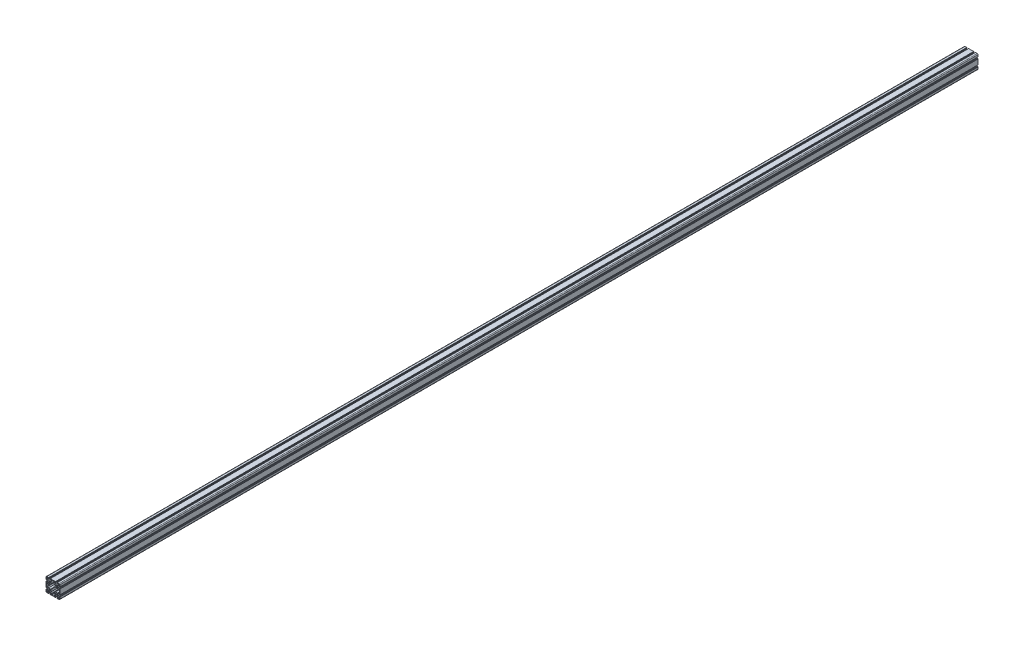
from build123d import *

# Parameters (mm, degrees)
SKETCH1_R           = 3.4
BOSS_EXTRUDE1_DEPTH = 5338


with BuildPart() as part:
    # Sketch1 → Boss-Extrude1 (new body)
    with BuildSketch(Plane.XY.offset(100)):
        with BuildLine():
            Line((37.78472507, 10.370402299), (32.802492023, 10.370402299))
            Line((32.802492023, 10.370402299), (28.48472507, 14.688169252))
            Line((28.48472507, 14.688169252), (28.48472507, 26.552635346))
            Line((28.48472507, 26.552635346), (32.802492023, 30.870402299))
            Line((32.802492023, 30.870402299), (37.78472507, 30.870402299))
            ThreePointArc((37.78472507, 30.870402299), (38.491831851, 30.57750908), (38.78472507, 29.870402299))
            Line((38.78472507, 29.870402299), (38.78472507, 28.220402299))
            ThreePointArc((38.78472507, 28.220402299), (38.491831851, 27.513295518), (37.78472507, 27.220402299))
            Line((37.78472507, 27.220402299), (36.28472507, 27.220402299))
            Line((36.28472507, 27.220402299), (36.28472507, 25.020402299))
            ThreePointArc((36.28472507, 25.020402299), (36.372593036, 24.808270264), (36.58472507, 24.720402299))
            Line((36.58472507, 24.720402299), (39.78472507, 24.720402299))
            Line((39.78472507, 24.720402299), (39.78472507, 25.520402299))
            ThreePointArc((39.78472507, 25.520402299), (39.843303714, 25.661823655), (39.98472507, 25.720402299))
            Line((39.98472507, 25.720402299), (40.78472507, 25.720402299))
            Line((40.78472507, 25.720402299), (40.78472507, 36.120402299))
            ThreePointArc((40.78472507, 36.120402299), (39.466705585, 39.302382814), (36.28472507, 40.620402299))
            Line((36.28472507, 40.620402299), (25.88472507, 40.620402299))
            Line((25.88472507, 40.620402299), (25.88472507, 39.820402299))
            ThreePointArc((25.88472507, 39.820402299), (25.826146426, 39.678980943), (25.68472507, 39.620402299))
            Line((25.68472507, 39.620402299), (24.88472507, 39.620402299))
            Line((24.88472507, 39.620402299), (24.88472507, 36.420402299))
            ThreePointArc((24.88472507, 36.420402299), (24.972593036, 36.208270264), (25.18472507, 36.120402299))
            Line((25.18472507, 36.120402299), (27.38472507, 36.120402299))
            Line((27.38472507, 36.120402299), (27.38472507, 37.620402299))
            ThreePointArc((27.38472507, 37.620402299), (27.677618289, 38.32750908), (28.38472507, 38.620402299))
            Line((28.38472507, 38.620402299), (30.03472507, 38.620402299))
            ThreePointArc((30.03472507, 38.620402299), (30.741831851, 38.32750908), (31.03472507, 37.620402299))
            Line((31.03472507, 37.620402299), (31.03472507, 32.638169252))
            Line((31.03472507, 32.638169252), (26.716958117, 28.320402299))
            Line((26.716958117, 28.320402299), (14.852492023, 28.320402299))
            Line((14.852492023, 28.320402299), (10.53472507, 32.638169252))
            Line((10.53472507, 32.638169252), (10.53472507, 37.620402299))
            ThreePointArc((10.53472507, 37.620402299), (10.827618289, 38.32750908), (11.53472507, 38.620402299))
            Line((11.53472507, 38.620402299), (13.18472507, 38.620402299))
            ThreePointArc((13.18472507, 38.620402299), (13.891831851, 38.32750908), (14.18472507, 37.620402299))
            Line((14.18472507, 37.620402299), (14.18472507, 36.120402299))
            Line((14.18472507, 36.120402299), (16.38472507, 36.120402299))
            ThreePointArc((16.38472507, 36.120402299), (16.596857104, 36.208270264), (16.68472507, 36.420402299))
            Line((16.68472507, 36.420402299), (16.68472507, 39.620402299))
            Line((16.68472507, 39.620402299), (15.88472507, 39.620402299))
            ThreePointArc((15.88472507, 39.620402299), (15.743303714, 39.678980943), (15.68472507, 39.820402299))
            Line((15.68472507, 39.820402299), (15.68472507, 40.620402299))
            Line((15.68472507, 40.620402299), (-14.11527493, 40.620402299))
            Line((-14.11527493, 40.620402299), (-14.11527493, 39.820402299))
            ThreePointArc((-14.11527493, 39.820402299), (-14.173853574, 39.678980943), (-14.31527493, 39.620402299))
            Line((-14.31527493, 39.620402299), (-15.11527493, 39.620402299))
            Line((-15.11527493, 39.620402299), (-15.11527493, 36.420402299))
            ThreePointArc((-15.11527493, 36.420402299), (-15.027406964, 36.208270264), (-14.81527493, 36.120402299))
            Line((-14.81527493, 36.120402299), (-12.61527493, 36.120402299))
            Line((-12.61527493, 36.120402299), (-12.61527493, 37.620402299))
            ThreePointArc((-12.61527493, 37.620402299), (-12.322381711, 38.32750908), (-11.61527493, 38.620402299))
            Line((-11.61527493, 38.620402299), (-9.96527493, 38.620402299))
            ThreePointArc((-9.96527493, 38.620402299), (-9.258168149, 38.32750908), (-8.96527493, 37.620402299))
            Line((-8.96527493, 37.620402299), (-8.96527493, 32.638169252))
            Line((-8.96527493, 32.638169252), (-13.283041883, 28.320402299))
            Line((-13.283041883, 28.320402299), (-25.147507977, 28.320402299))
            Line((-25.147507977, 28.320402299), (-29.46527493, 32.638169252))
            Line((-29.46527493, 32.638169252), (-29.46527493, 37.620402299))
            ThreePointArc((-29.46527493, 37.620402299), (-29.172381711, 38.32750908), (-28.46527493, 38.620402299))
            Line((-28.46527493, 38.620402299), (-26.81527493, 38.620402299))
            ThreePointArc((-26.81527493, 38.620402299), (-26.108168149, 38.32750908), (-25.81527493, 37.620402299))
            Line((-25.81527493, 37.620402299), (-25.81527493, 36.120402299))
            Line((-25.81527493, 36.120402299), (-23.61527493, 36.120402299))
            ThreePointArc((-23.61527493, 36.120402299), (-23.403142896, 36.208270264), (-23.31527493, 36.420402299))
            Line((-23.31527493, 36.420402299), (-23.31527493, 39.620402299))
            Line((-23.31527493, 39.620402299), (-24.11527493, 39.620402299))
            ThreePointArc((-24.11527493, 39.620402299), (-24.256696286, 39.678980943), (-24.31527493, 39.820402299))
            Line((-24.31527493, 39.820402299), (-24.31527493, 40.620402299))
            Line((-24.31527493, 40.620402299), (-34.71527493, 40.620402299))
            ThreePointArc((-34.71527493, 40.620402299), (-37.897255445, 39.302382814), (-39.21527493, 36.120402299))
            Line((-39.21527493, 36.120402299), (-39.21527493, 25.720402299))
            Line((-39.21527493, 25.720402299), (-38.41527493, 25.720402299))
            ThreePointArc((-38.41527493, 25.720402299), (-38.273853574, 25.661823655), (-38.21527493, 25.520402299))
            Line((-38.21527493, 25.520402299), (-38.21527493, 24.720402299))
            Line((-38.21527493, 24.720402299), (-35.01527493, 24.720402299))
            ThreePointArc((-35.01527493, 24.720402299), (-34.803142896, 24.808270264), (-34.71527493, 25.020402299))
            Line((-34.71527493, 25.020402299), (-34.71527493, 27.220402299))
            Line((-34.71527493, 27.220402299), (-36.21527493, 27.220402299))
            ThreePointArc((-36.21527493, 27.220402299), (-36.922381711, 27.513295518), (-37.21527493, 28.220402299))
            Line((-37.21527493, 28.220402299), (-37.21527493, 29.870402299))
            ThreePointArc((-37.21527493, 29.870402299), (-36.922381711, 30.57750908), (-36.21527493, 30.870402299))
            Line((-36.21527493, 30.870402299), (-31.233041883, 30.870402299))
            Line((-31.233041883, 30.870402299), (-26.91527493, 26.552635346))
            Line((-26.91527493, 26.552635346), (-26.91527493, 14.688169252))
            Line((-26.91527493, 14.688169252), (-31.233041883, 10.370402299))
            Line((-31.233041883, 10.370402299), (-36.21527493, 10.370402299))
            ThreePointArc((-36.21527493, 10.370402299), (-36.922381711, 10.663295518), (-37.21527493, 11.370402299))
            Line((-37.21527493, 11.370402299), (-37.21527493, 13.020402299))
            ThreePointArc((-37.21527493, 13.020402299), (-36.922381711, 13.72750908), (-36.21527493, 14.020402299))
            Line((-36.21527493, 14.020402299), (-34.71527493, 14.020402299))
            Line((-34.71527493, 14.020402299), (-34.71527493, 16.220402299))
            ThreePointArc((-34.71527493, 16.220402299), (-34.803142896, 16.432534333), (-35.01527493, 16.520402299))
            Line((-35.01527493, 16.520402299), (-38.21527493, 16.520402299))
            Line((-38.21527493, 16.520402299), (-38.21527493, 15.720402299))
            ThreePointArc((-38.21527493, 15.720402299), (-38.273853574, 15.578980943), (-38.41527493, 15.520402299))
            Line((-38.41527493, 15.520402299), (-39.21527493, 15.520402299))
            Line((-39.21527493, 15.520402299), (-39.21527493, -14.279597701))
            Line((-39.21527493, -14.279597701), (-38.41527493, -14.279597701))
            ThreePointArc((-38.41527493, -14.279597701), (-38.273853574, -14.338176345), (-38.21527493, -14.479597701))
            Line((-38.21527493, -14.479597701), (-38.21527493, -15.279597701))
            Line((-38.21527493, -15.279597701), (-35.01527493, -15.279597701))
            ThreePointArc((-35.01527493, -15.279597701), (-34.803142896, -15.191729736), (-34.71527493, -14.979597701))
            Line((-34.71527493, -14.979597701), (-34.71527493, -12.779597701))
            Line((-34.71527493, -12.779597701), (-36.21527493, -12.779597701))
            ThreePointArc((-36.21527493, -12.779597701), (-36.922381711, -12.486704482), (-37.21527493, -11.779597701))
            Line((-37.21527493, -11.779597701), (-37.21527493, -10.129597701))
            ThreePointArc((-37.21527493, -10.129597701), (-36.922381711, -9.42249092), (-36.21527493, -9.129597701))
            Line((-36.21527493, -9.129597701), (-31.233041883, -9.129597701))
            Line((-31.233041883, -9.129597701), (-26.91527493, -13.447364654))
            Line((-26.91527493, -13.447364654), (-26.91527493, -25.311830748))
            Line((-26.91527493, -25.311830748), (-31.233041883, -29.629597701))
            Line((-31.233041883, -29.629597701), (-36.21527493, -29.629597701))
            ThreePointArc((-36.21527493, -29.629597701), (-36.922381711, -29.336704482), (-37.21527493, -28.629597701))
            Line((-37.21527493, -28.629597701), (-37.21527493, -26.979597701))
            ThreePointArc((-37.21527493, -26.979597701), (-36.922381711, -26.27249092), (-36.21527493, -25.979597701))
            Line((-36.21527493, -25.979597701), (-34.71527493, -25.979597701))
            Line((-34.71527493, -25.979597701), (-34.71527493, -23.779597701))
            ThreePointArc((-34.71527493, -23.779597701), (-34.803142896, -23.567465667), (-35.01527493, -23.479597701))
            Line((-35.01527493, -23.479597701), (-38.21527493, -23.479597701))
            Line((-38.21527493, -23.479597701), (-38.21527493, -24.279597701))
            ThreePointArc((-38.21527493, -24.279597701), (-38.273853574, -24.421019057), (-38.41527493, -24.479597701))
            Line((-38.41527493, -24.479597701), (-39.21527493, -24.479597701))
            Line((-39.21527493, -24.479597701), (-39.21527493, -34.879597701))
            ThreePointArc((-39.21527493, -34.879597701), (-37.897255445, -38.061578216), (-34.71527493, -39.379597701))
            Line((-34.71527493, -39.379597701), (-24.31527493, -39.379597701))
            Line((-24.31527493, -39.379597701), (-24.31527493, -38.579597701))
            ThreePointArc((-24.31527493, -38.579597701), (-24.256696286, -38.438176345), (-24.11527493, -38.379597701))
            Line((-24.11527493, -38.379597701), (-23.31527493, -38.379597701))
            Line((-23.31527493, -38.379597701), (-23.31527493, -35.179597701))
            ThreePointArc((-23.31527493, -35.179597701), (-23.403142896, -34.967465667), (-23.61527493, -34.879597701))
            Line((-23.61527493, -34.879597701), (-25.81527493, -34.879597701))
            Line((-25.81527493, -34.879597701), (-25.81527493, -36.379597701))
            ThreePointArc((-25.81527493, -36.379597701), (-26.108168149, -37.086704482), (-26.81527493, -37.379597701))
            Line((-26.81527493, -37.379597701), (-28.46527493, -37.379597701))
            ThreePointArc((-28.46527493, -37.379597701), (-29.172381711, -37.086704482), (-29.46527493, -36.379597701))
            Line((-29.46527493, -36.379597701), (-29.46527493, -31.397364654))
            Line((-29.46527493, -31.397364654), (-25.147507977, -27.079597701))
            Line((-25.147507977, -27.079597701), (-13.283041883, -27.079597701))
            Line((-13.283041883, -27.079597701), (-8.96527493, -31.397364654))
            Line((-8.96527493, -31.397364654), (-8.96527493, -36.379597701))
            ThreePointArc((-8.96527493, -36.379597701), (-9.258168149, -37.086704482), (-9.96527493, -37.379597701))
            Line((-9.96527493, -37.379597701), (-11.61527493, -37.379597701))
            ThreePointArc((-11.61527493, -37.379597701), (-12.322381711, -37.086704482), (-12.61527493, -36.379597701))
            Line((-12.61527493, -36.379597701), (-12.61527493, -34.879597701))
            Line((-12.61527493, -34.879597701), (-14.81527493, -34.879597701))
            ThreePointArc((-14.81527493, -34.879597701), (-15.027406964, -34.967465667), (-15.11527493, -35.179597701))
            Line((-15.11527493, -35.179597701), (-15.11527493, -38.379597701))
            Line((-15.11527493, -38.379597701), (-14.31527493, -38.379597701))
            ThreePointArc((-14.31527493, -38.379597701), (-14.173853574, -38.438176345), (-14.11527493, -38.579597701))
            Line((-14.11527493, -38.579597701), (-14.11527493, -39.379597701))
            Line((-14.11527493, -39.379597701), (15.68472507, -39.379597701))
            Line((15.68472507, -39.379597701), (15.68472507, -38.579597701))
            ThreePointArc((15.68472507, -38.579597701), (15.743303714, -38.438176345), (15.88472507, -38.379597701))
            Line((15.88472507, -38.379597701), (16.68472507, -38.379597701))
            Line((16.68472507, -38.379597701), (16.68472507, -35.179597701))
            ThreePointArc((16.68472507, -35.179597701), (16.596857104, -34.967465667), (16.38472507, -34.879597701))
            Line((16.38472507, -34.879597701), (14.18472507, -34.879597701))
            Line((14.18472507, -34.879597701), (14.18472507, -36.379597701))
            ThreePointArc((14.18472507, -36.379597701), (13.891831851, -37.086704482), (13.18472507, -37.379597701))
            Line((13.18472507, -37.379597701), (11.53472507, -37.379597701))
            ThreePointArc((11.53472507, -37.379597701), (10.827618289, -37.086704482), (10.53472507, -36.379597701))
            Line((10.53472507, -36.379597701), (10.53472507, -31.397364654))
            Line((10.53472507, -31.397364654), (14.852492023, -27.079597701))
            Line((14.852492023, -27.079597701), (26.716958117, -27.079597701))
            Line((26.716958117, -27.079597701), (31.03472507, -31.397364654))
            Line((31.03472507, -31.397364654), (31.03472507, -36.379597701))
            ThreePointArc((31.03472507, -36.379597701), (30.741831851, -37.086704482), (30.03472507, -37.379597701))
            Line((30.03472507, -37.379597701), (28.38472507, -37.379597701))
            ThreePointArc((28.38472507, -37.379597701), (27.677618289, -37.086704482), (27.38472507, -36.379597701))
            Line((27.38472507, -36.379597701), (27.38472507, -34.879597701))
            Line((27.38472507, -34.879597701), (25.18472507, -34.879597701))
            ThreePointArc((25.18472507, -34.879597701), (24.972593036, -34.967465667), (24.88472507, -35.179597701))
            Line((24.88472507, -35.179597701), (24.88472507, -38.379597701))
            Line((24.88472507, -38.379597701), (25.68472507, -38.379597701))
            ThreePointArc((25.68472507, -38.379597701), (25.826146426, -38.438176345), (25.88472507, -38.579597701))
            Line((25.88472507, -38.579597701), (25.88472507, -39.379597701))
            Line((25.88472507, -39.379597701), (36.28472507, -39.379597701))
            ThreePointArc((36.28472507, -39.379597701), (39.466705585, -38.061578216), (40.78472507, -34.879597701))
            Line((40.78472507, -34.879597701), (40.78472507, -24.479597701))
            Line((40.78472507, -24.479597701), (39.98472507, -24.479597701))
            ThreePointArc((39.98472507, -24.479597701), (39.843303714, -24.421019057), (39.78472507, -24.279597701))
            Line((39.78472507, -24.279597701), (39.78472507, -23.479597701))
            Line((39.78472507, -23.479597701), (36.58472507, -23.479597701))
            ThreePointArc((36.58472507, -23.479597701), (36.372593036, -23.567465667), (36.28472507, -23.779597701))
            Line((36.28472507, -23.779597701), (36.28472507, -25.979597701))
            Line((36.28472507, -25.979597701), (37.78472507, -25.979597701))
            ThreePointArc((37.78472507, -25.979597701), (38.491831851, -26.27249092), (38.78472507, -26.979597701))
            Line((38.78472507, -26.979597701), (38.78472507, -28.629597701))
            ThreePointArc((38.78472507, -28.629597701), (38.491831851, -29.336704482), (37.78472507, -29.629597701))
            Line((37.78472507, -29.629597701), (32.802492023, -29.629597701))
            Line((32.802492023, -29.629597701), (28.48472507, -25.311830748))
            Line((28.48472507, -25.311830748), (28.48472507, -13.447364654))
            Line((28.48472507, -13.447364654), (32.802492023, -9.129597701))
            Line((32.802492023, -9.129597701), (37.78472507, -9.129597701))
            ThreePointArc((37.78472507, -9.129597701), (38.491831851, -9.42249092), (38.78472507, -10.129597701))
            Line((38.78472507, -10.129597701), (38.78472507, -11.779597701))
            ThreePointArc((38.78472507, -11.779597701), (38.491831851, -12.486704482), (37.78472507, -12.779597701))
            Line((37.78472507, -12.779597701), (36.28472507, -12.779597701))
            Line((36.28472507, -12.779597701), (36.28472507, -14.979597701))
            ThreePointArc((36.28472507, -14.979597701), (36.372593036, -15.191729736), (36.58472507, -15.279597701))
            Line((36.58472507, -15.279597701), (39.78472507, -15.279597701))
            Line((39.78472507, -15.279597701), (39.78472507, -14.479597701))
            ThreePointArc((39.78472507, -14.479597701), (39.843303714, -14.338176345), (39.98472507, -14.279597701))
            Line((39.98472507, -14.279597701), (40.78472507, -14.279597701))
            Line((40.78472507, -14.279597701), (40.78472507, 15.520402299))
            Line((40.78472507, 15.520402299), (39.98472507, 15.520402299))
            ThreePointArc((39.98472507, 15.520402299), (39.843303714, 15.578980943), (39.78472507, 15.720402299))
            Line((39.78472507, 15.720402299), (39.78472507, 16.520402299))
            Line((39.78472507, 16.520402299), (36.58472507, 16.520402299))
            ThreePointArc((36.58472507, 16.520402299), (36.372593036, 16.432534333), (36.28472507, 16.220402299))
            Line((36.28472507, 16.220402299), (36.28472507, 14.020402299))
            Line((36.28472507, 14.020402299), (37.78472507, 14.020402299))
            ThreePointArc((37.78472507, 14.020402299), (38.491831851, 13.72750908), (38.78472507, 13.020402299))
            Line((38.78472507, 13.020402299), (38.78472507, 11.370402299))
            ThreePointArc((38.78472507, 11.370402299), (38.491831851, 10.663295518), (37.78472507, 10.370402299))
        make_face()
        with Locations(Location((-19.21527493, -19.379597701, 0), (0, 0, 180))):
            Circle(SKETCH1_R, mode=Mode.SUBTRACT)
        with Locations(Location((20.78472507, -19.379597701, 0), (0, 0, 180))):
            Circle(SKETCH1_R, mode=Mode.SUBTRACT)
        with Locations(Location((20.78472507, 20.620402299, 0), (0, 0, 180))):
            Circle(SKETCH1_R, mode=Mode.SUBTRACT)
        with Locations(Location((-19.21527493, 20.620402299, 0), (0, 0, 180))):
            Circle(SKETCH1_R, mode=Mode.SUBTRACT)
        with BuildLine():
            Line((-29.61172154, 8.456188736), (-25.147507977, 12.920402299))
            Line((-25.147507977, 12.920402299), (-14.01527493, 12.920402299))
            ThreePointArc((-14.01527493, 12.920402299), (-12.247507977, 13.652635346), (-11.51527493, 15.420402299))
            Line((-11.51527493, 15.420402299), (-11.51527493, 26.552635346))
            Line((-11.51527493, 26.552635346), (-7.051061368, 31.016848908))
            ThreePointArc((-7.051061368, 31.016848908), (-6.617515865, 31.665695606), (-6.46527493, 32.431062471))
            Line((-6.46527493, 32.431062471), (-6.46527493, 37.420402299))
            ThreePointArc((-6.46527493, 37.420402299), (-6.172381711, 38.12750908), (-5.46527493, 38.420402299))
            Line((-5.46527493, 38.420402299), (7.03472507, 38.420402299))
            ThreePointArc((7.03472507, 38.420402299), (7.741831851, 38.12750908), (8.03472507, 37.420402299))
            Line((8.03472507, 37.420402299), (8.03472507, 32.431062471))
            ThreePointArc((8.03472507, 32.431062471), (8.186966005, 31.665695606), (8.620511508, 31.016848908))
            Line((8.620511508, 31.016848908), (13.08472507, 26.552635346))
            Line((13.08472507, 26.552635346), (13.08472507, 15.420402299))
            ThreePointArc((13.08472507, 15.420402299), (13.816958117, 13.652635346), (15.58472507, 12.920402299))
            Line((15.58472507, 12.920402299), (26.716958117, 12.920402299))
            Line((26.716958117, 12.920402299), (31.181171679, 8.456188736))
            ThreePointArc((31.181171679, 8.456188736), (31.830018377, 8.022643234), (32.595385242, 7.870402299))
            Line((32.595385242, 7.870402299), (37.58472507, 7.870402299))
            ThreePointArc((37.58472507, 7.870402299), (38.291831851, 7.57750908), (38.58472507, 6.870402299))
            Line((38.58472507, 6.870402299), (38.58472507, -5.629597701))
            ThreePointArc((38.58472507, -5.629597701), (38.291831851, -6.336704482), (37.58472507, -6.629597701))
            Line((37.58472507, -6.629597701), (32.595385242, -6.629597701))
            ThreePointArc((32.595385242, -6.629597701), (31.830018377, -6.781838636), (31.181171679, -7.215384139))
            Line((31.181171679, -7.215384139), (26.716958117, -11.679597701))
            Line((26.716958117, -11.679597701), (15.58472507, -11.679597701))
            ThreePointArc((15.58472507, -11.679597701), (13.816958117, -12.411830748), (13.08472507, -14.179597701))
            Line((13.08472507, -14.179597701), (13.08472507, -24.483403623))
            ThreePointArc((13.08472507, -24.483403623), (12.932484135, -25.248770488), (12.498938632, -25.897617186))
            Line((12.498938632, -25.897617186), (8.620511508, -29.776044311))
            ThreePointArc((8.620511508, -29.776044311), (8.186966005, -30.424891008), (8.03472507, -31.190257873))
            Line((8.03472507, -31.190257873), (8.03472507, -36.179597701))
            ThreePointArc((8.03472507, -36.179597701), (7.741831851, -36.886704482), (7.03472507, -37.179597701))
            Line((7.03472507, -37.179597701), (-5.46527493, -37.179597701))
            ThreePointArc((-5.46527493, -37.179597701), (-6.172381711, -36.886704482), (-6.46527493, -36.179597701))
            Line((-6.46527493, -36.179597701), (-6.46527493, -31.190257873))
            ThreePointArc((-6.46527493, -31.190257873), (-6.617515865, -30.424891008), (-7.051061368, -29.776044311))
            Line((-7.051061368, -29.776044311), (-11.51527493, -25.311830748))
            Line((-11.51527493, -25.311830748), (-11.51527493, -14.179597701))
            ThreePointArc((-11.51527493, -14.179597701), (-12.247507977, -12.411830748), (-14.01527493, -11.679597701))
            Line((-14.01527493, -11.679597701), (-25.147507977, -11.679597701))
            Line((-25.147507977, -11.679597701), (-29.61172154, -7.215384139))
            ThreePointArc((-29.61172154, -7.215384139), (-30.260568237, -6.781838636), (-31.025935102, -6.629597701))
            Line((-31.025935102, -6.629597701), (-36.01527493, -6.629597701))
            ThreePointArc((-36.01527493, -6.629597701), (-36.722381711, -6.336704482), (-37.01527493, -5.629597701))
            Line((-37.01527493, -5.629597701), (-37.01527493, 6.870402299))
            ThreePointArc((-37.01527493, 6.870402299), (-36.722381711, 7.57750908), (-36.01527493, 7.870402299))
            Line((-36.01527493, 7.870402299), (-31.025935102, 7.870402299))
            ThreePointArc((-31.025935102, 7.870402299), (-30.260568237, 8.022643234), (-29.61172154, 8.456188736))
        make_face(mode=Mode.SUBTRACT)
        with BuildLine():
            Line((-35.21927493, 39.124402299), (-31.96527493, 39.124402299))
            ThreePointArc((-31.96527493, 39.124402299), (-31.258168149, 38.83150908), (-30.96527493, 38.124402299))
            Line((-30.96527493, 38.124402299), (-30.96527493, 33.370402299))
            ThreePointArc((-30.96527493, 33.370402299), (-31.258168149, 32.663295518), (-31.96527493, 32.370402299))
            Line((-31.96527493, 32.370402299), (-36.71927493, 32.370402299))
            ThreePointArc((-36.71927493, 32.370402299), (-37.426381711, 32.663295518), (-37.71927493, 33.370402299))
            Line((-37.71927493, 33.370402299), (-37.71927493, 36.624402299))
            ThreePointArc((-37.71927493, 36.624402299), (-36.987041883, 38.392169252), (-35.21927493, 39.124402299))
        make_face(mode=Mode.SUBTRACT)
        with BuildLine():
            Line((36.78872507, -37.883597701), (33.53472507, -37.883597701))
            ThreePointArc((33.53472507, -37.883597701), (32.827618289, -37.590704482), (32.53472507, -36.883597701))
            Line((32.53472507, -36.883597701), (32.53472507, -32.129597701))
            ThreePointArc((32.53472507, -32.129597701), (32.827618289, -31.42249092), (33.53472507, -31.129597701))
            Line((33.53472507, -31.129597701), (38.28872507, -31.129597701))
            ThreePointArc((38.28872507, -31.129597701), (38.995831851, -31.42249092), (39.28872507, -32.129597701))
            Line((39.28872507, -32.129597701), (39.28872507, -35.383597701))
            ThreePointArc((39.28872507, -35.383597701), (38.556492023, -37.151364654), (36.78872507, -37.883597701))
        make_face(mode=Mode.SUBTRACT)
        with BuildLine():
            Line((-37.71927493, -35.383597701), (-37.71927493, -32.129597701))
            ThreePointArc((-37.71927493, -32.129597701), (-37.426381711, -31.42249092), (-36.71927493, -31.129597701))
            Line((-36.71927493, -31.129597701), (-31.96527493, -31.129597701))
            ThreePointArc((-31.96527493, -31.129597701), (-31.258168149, -31.42249092), (-30.96527493, -32.129597701))
            Line((-30.96527493, -32.129597701), (-30.96527493, -36.883597701))
            ThreePointArc((-30.96527493, -36.883597701), (-31.258168149, -37.590704482), (-31.96527493, -37.883597701))
            Line((-31.96527493, -37.883597701), (-35.21927493, -37.883597701))
            ThreePointArc((-35.21927493, -37.883597701), (-36.987041883, -37.151364654), (-37.71927493, -35.383597701))
        make_face(mode=Mode.SUBTRACT)
        with BuildLine():
            Line((39.28872507, 36.624402299), (39.28872507, 33.370402299))
            ThreePointArc((39.28872507, 33.370402299), (38.995831851, 32.663295518), (38.28872507, 32.370402299))
            Line((38.28872507, 32.370402299), (33.53472507, 32.370402299))
            ThreePointArc((33.53472507, 32.370402299), (32.827618289, 32.663295518), (32.53472507, 33.370402299))
            Line((32.53472507, 33.370402299), (32.53472507, 38.124402299))
            ThreePointArc((32.53472507, 38.124402299), (32.827618289, 38.83150908), (33.53472507, 39.124402299))
            Line((33.53472507, 39.124402299), (36.78872507, 39.124402299))
            ThreePointArc((36.78872507, 39.124402299), (38.556492023, 38.392169252), (39.28872507, 36.624402299))
        make_face(mode=Mode.SUBTRACT)
    extrude(amount=-BOSS_EXTRUDE1_DEPTH)


solid = part.part
